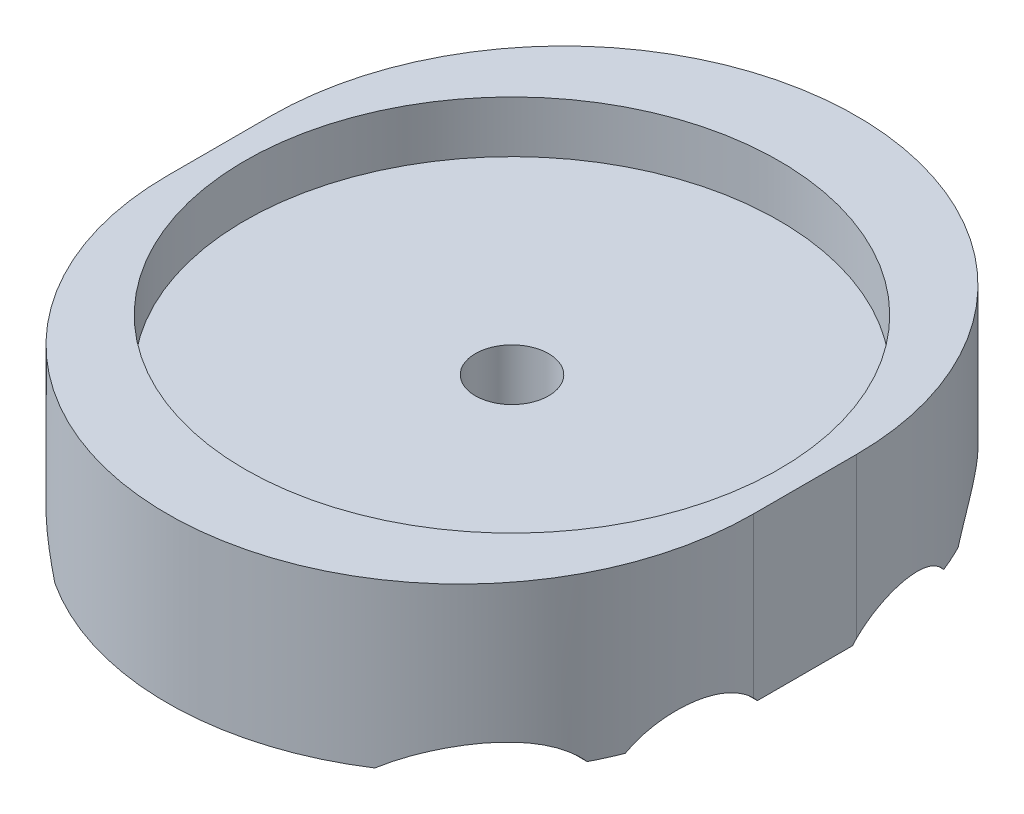
SolidWorks part; units mm, degrees
material "45"
ref_plane "前视基准面" through (0, 0, 0) normal (0, 0, 1) x (1, 0, 0)
ref_plane "上视基准面" through (0, 0, 0) normal (0, 1, 0) x (1, 0, 0)
ref_plane "右视基准面" through (0, 0, 0) normal (1, 0, 0) x (0, 0, -1)
sketch "草图1" plane through (0, 0, 0) normal (0, 1, 0) x (1, 0, 0)
  line L0 (0, 6) -> (0, -6) construction
  line L5 (0, 0) -> (34, 0) construction
  line L6 (34, -6) -> (34, 6)
  line L7 (-34, -6) -> (-34, 6)
  arc A0 (34, 6) -> (-34, 6) centre (0, 6) ccw
  arc A1 (34, -6) -> (-34, -6) centre (0, -6) cw
  point P4 (0, 40)
  point P11 (-34, 0)
  point P12 (0, -40)
  dimension "D1" = 34
  dimension "D2" = 34
  dimension "D3" = 6
  dimension "D4" = 80
extrude "凸台-拉伸1" add sketch "草图1" along normal blind 19
sketch "草图2" plane through (0, 19, 0) normal (0, 1, 0) x (1, 0, 0)
  circle A0 centre (0, 0) radius 31
  dimension "D1" = 62
extrude "切除-拉伸1" cut sketch "草图2" against normal blind 6
hole_wizard "M10 螺纹孔1" positions "草图3" profile "草图4" tap size "M10" standard "GB"
sketch "草图3" plane through (0, 13, 0) normal (0, 1, 0) x (1, 0, 0)
  point P0 (0, 0)
sketch "草图4" plane through (0, 13, 0) normal (1, 0, 0) x (0, 0, 1)
  line L0 (0, 0) -> (0, 8.5537)
  line L1 (0, 8.5537) -> (4.25, 6)
  line L2 (4.25, 6) -> (4.25, 0)
  line L5 (4.25, 0) -> (0, 0)
  line L10 (0, 8.5537) -> (-4.25, 6) construction
  line L11 (0, -6.35) -> (0, 107.95) construction
  dimension "螺纹孔钻头直径" = 8.5
  dimension "螺纹孔钻头深度" = 6
  dimension "导头角度" = 118
cosmetic thread "孔螺蚊线1" parameters "D1"=20, "D2"=10
sketch "草图5" plane through (0, 0, 0) normal (1, 0, 0) x (0, 0, -1)
  line L0 (0, 0) -> (0, 19) construction
  line L1 (-6, 19) -> (6, 19) construction
  line L2 (-40, 0) -> (-6, 0) construction
  circle A0 centre (-28, -5.5) radius 8.5
  circle A1 centre (-12, -5.5) radius 8.5
  circle A2 centre (12, -5.5) radius 8.5
  circle A3 centre (28, -5.5) radius 8.5
  dimension "D1" = 17
  dimension "D2" = 24
  dimension "D3" = 56
  dimension "D4" = 5.5
extrude "切除-拉伸2" cut sketch "草图5" against normal through all both and the other way through all contours A3 A2 | A2 A3 | A0 A1 | A1 A0
